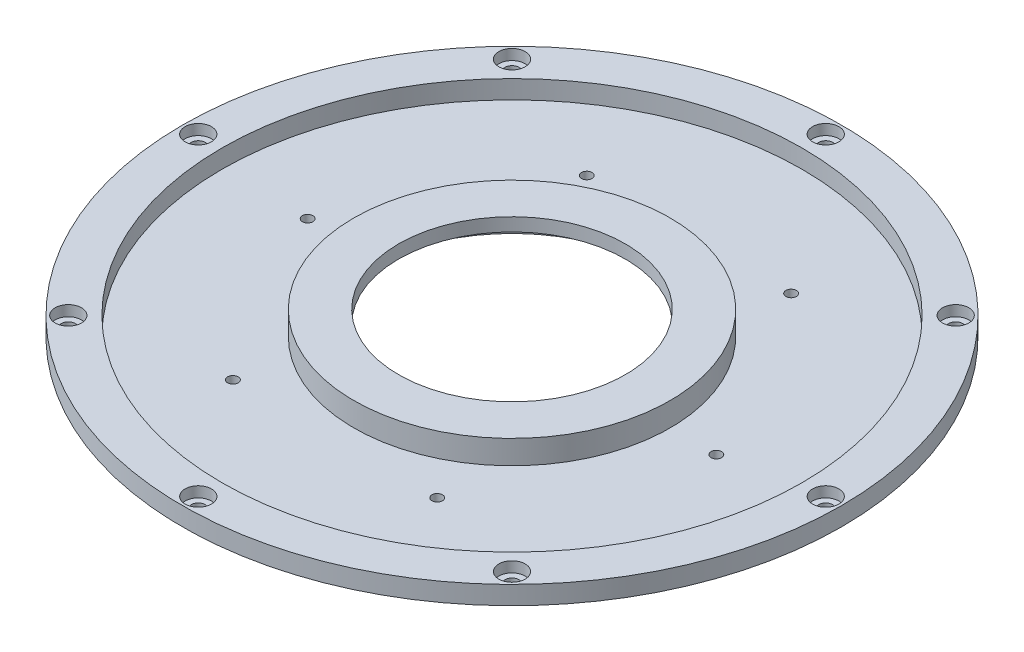
from build123d import *

# Parameters (mm, degrees)
SKETCH2_R          = 2.65
CUT_EXTRUDE1_DEPTH = 10
SKETCH3_R          = 5
CUT_EXTRUDE3_DEPTH = 4
SKETCH4_R          = 2
CUT_EXTRUDE4_DEPTH = 20


with BuildPart() as part:
    # Sketch1 → Revolve1 (revolve)
    with BuildSketch(Plane.XY):
        Polygon((-125, 132), (-115, 132), (-115, 127), (-55, 127), (-55, 136), (-43, 136), (-43, 141), (-60, 141), (-60, 132), (-110, 132), (-110, 139), (-125, 139), align=None)
    revolve(axis=Axis((0, 0, 0), (0, -1, 0)))

    # Sketch2 → Cut-Extrude1 (cut)
    with BuildSketch(Plane(origin=(0, 139, 0), x_dir=(1, 0, 0), z_dir=(0, 1, 0))):
        with Locations(Location((0, 119, 0), (0, 0, 180))):
            Circle(SKETCH2_R)
        with Locations(Location((84.145706961, 84.145706961, 0), (0, 0, 180))):
            Circle(SKETCH2_R)
        with Locations(Location((119, 0, 0), (0, 0, 180))):
            Circle(SKETCH2_R)
        with Locations(Location((84.145706961, -84.145706961, 0), (0, 0, 180))):
            Circle(SKETCH2_R)
        with Locations(Location((0, -119, 0), (0, 0, 180))):
            Circle(SKETCH2_R)
        with Locations(Location((-84.145706961, -84.145706961, 0), (0, 0, 180))):
            Circle(SKETCH2_R)
        with Locations(Location((-119, 0, 0), (0, 0, 180))):
            Circle(SKETCH2_R)
        with Locations(Location((-84.145706961, 84.145706961, 0), (0, 0, 180))):
            Circle(SKETCH2_R)
    extrude(amount=-CUT_EXTRUDE1_DEPTH, mode=Mode.SUBTRACT)

    # Sketch3 → Cut-Extrude3 (cut)
    with BuildSketch(Plane(origin=(0, 139, 0), x_dir=(1, 0, 0), z_dir=(0, 1, 0))):
        with Locations(Location((0, 119, 0), (0, 0, 180))):
            Circle(SKETCH3_R)
        with Locations(Location((84.145706961, 84.145706961, 0), (0, 0, 180))):
            Circle(SKETCH3_R)
        with Locations(Location((119, 0, 0), (0, 0, 180))):
            Circle(SKETCH3_R)
        with Locations(Location((84.145706961, -84.145706961, 0), (0, 0, 180))):
            Circle(SKETCH3_R)
        with Locations(Location((0, -119, 0), (0, 0, 180))):
            Circle(SKETCH3_R)
        with Locations(Location((-84.145706961, -84.145706961, 0), (0, 0, 180))):
            Circle(SKETCH3_R)
        with Locations(Location((-119, 0, 0), (0, 0, 180))):
            Circle(SKETCH3_R)
        with Locations(Location((-84.145706961, 84.145706961, 0), (0, 0, 180))):
            Circle(SKETCH3_R)
    extrude(amount=-CUT_EXTRUDE3_DEPTH, mode=Mode.SUBTRACT)

    # Sketch4 → Cut-Extrude4 (cut)
    with BuildSketch(Plane(origin=(0, 132, 0), x_dir=(1, 0, 0), z_dir=(0, 1, 0))):
        with Locations(Location((77.5, 0, 0), (0, 0, 180))):
            Circle(SKETCH4_R)
        with Locations(Location((38.75, -67.116968793, 0), (0, 0, 180))):
            Circle(SKETCH4_R)
        with Locations(Location((-38.75, -67.116968793, 0), (0, 0, 180))):
            Circle(SKETCH4_R)
        with Locations(Location((-77.5, 0, 0), (0, 0, 180))):
            Circle(SKETCH4_R)
        with Locations(Location((-38.75, 67.116968793, 0), (0, 0, 180))):
            Circle(SKETCH4_R)
        with Locations(Location((38.75, 67.116968793, 0), (0, 0, 180))):
            Circle(SKETCH4_R)
    extrude(amount=-CUT_EXTRUDE4_DEPTH, mode=Mode.SUBTRACT)


solid = part.part
